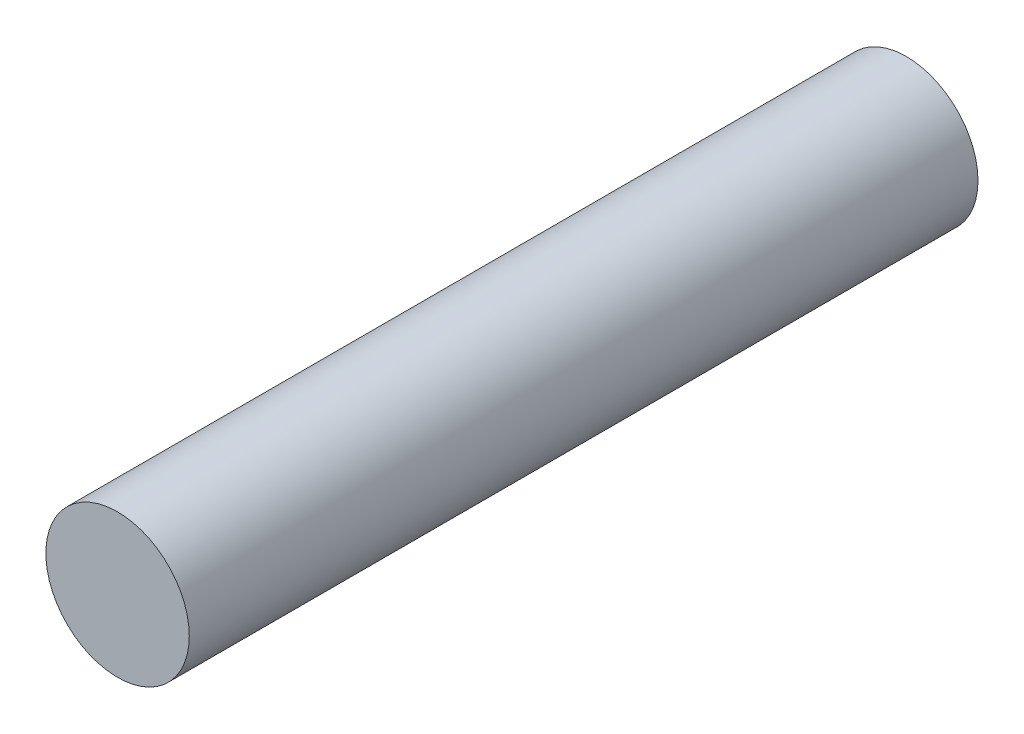
from build123d import *

# Parameters (mm, degrees)
SKETCH1_R           = 5
BOSS_EXTRUDE1_DEPTH = 55


with BuildPart() as part:
    # Sketch1 → Boss-Extrude1 (new body)
    with BuildSketch(Plane.XY):
        Circle(SKETCH1_R)
    extrude(amount=BOSS_EXTRUDE1_DEPTH)


solid = part.part
